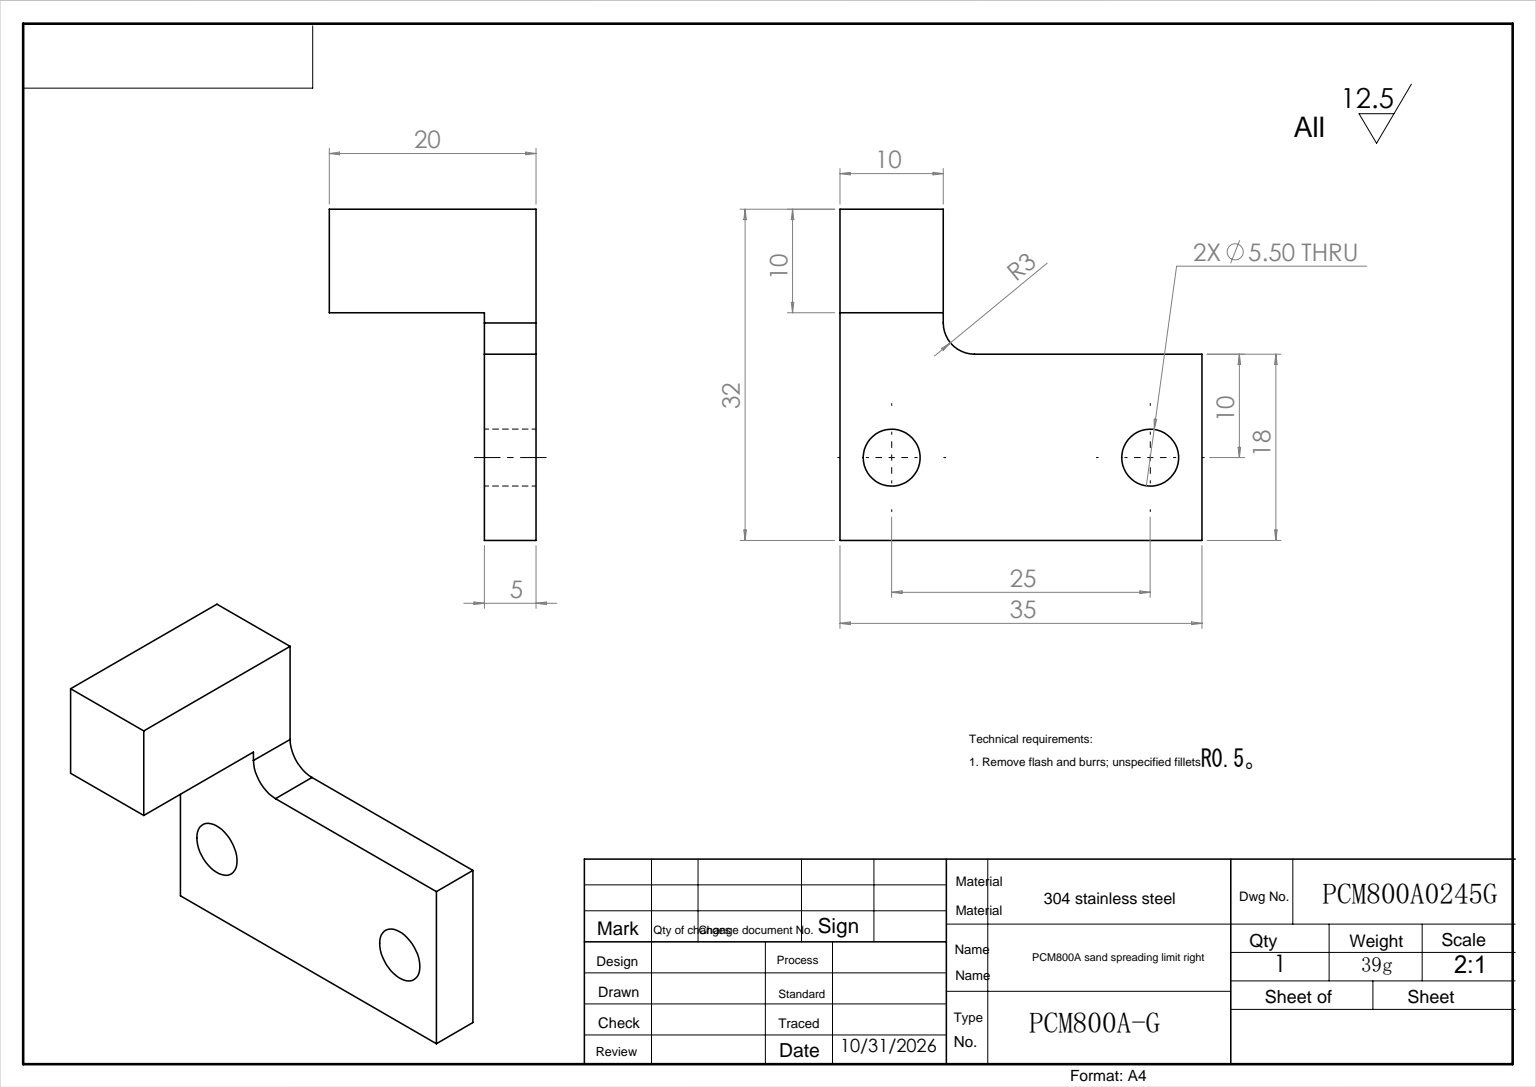
SolidWorks part; units mm, degrees
ref_plane "前视基准面" through (0, 0, 0) normal (0, 0, 1) x (1, 0, 0)
ref_plane "上视基准面" through (0, 0, 0) normal (0, 1, 0) x (1, 0, 0)
ref_plane "右视基准面" through (0, 0, 0) normal (1, 0, 0) x (0, 0, -1)
sketch "草图1" plane through (0, 0, 0) normal (0, 0, 1) x (1, 0, 0)
  line L1 (0, 0) -> (35, 0)
  line L2 (0, 0) -> (0, 22)
  line L3 (13, 18) -> (35, 18)
  line L4 (35, 0) -> (35, 18)
  line L7 (0, 22) -> (10, 22)
  line L8 (10, 21) -> (10, 22)
  arc A0 (13, 18) -> (10, 21) centre (13, 21) cw
  dimension "D4" = 3
  dimension "D1" = 18
  dimension "D2" = 35
  dimension "D3" = 22
  dimension "D5" = 10
  dimension "D6" = 1
extrude "凸台-拉伸1" add sketch "草图1" along normal blind 5
sketch "草图5" plane through (0, 0, 0) normal (0, 0, -1) x (-1, 0, 0)
  line L1 (0, 22) -> (-10, 22)
  line L2 (0, 22) -> (0, 32)
  line L3 (0, 32) -> (-10, 32)
  line L4 (-10, 22) -> (-10, 32)
  dimension "D1" = 10
  dimension "D2" = 10
extrude "凸台-拉伸3" add sketch "草图5" against normal blind 20
sketch "草图4" plane through (0, 0, 0) normal (0, 0, -1) x (-1, 0, 0)
  line L1 (-17.5, 0) -> (-17.5, 27.8202) construction
  line L2 (0, 0) -> (-35, 0) construction
  line L3 (0, 32) -> (-10, 32) construction
  circle A0 centre (-30, 8) radius 2.75
  circle A1 centre (-5, 8) radius 2.75
  dimension "D3" = 25
  dimension "D5" = 5.5
  dimension "D6" = 5.5
  dimension "D1" = 24
  dimension "D2" = 24
  dimension "D4" = 12.5
extrude "切除-拉伸1" cut sketch "草图4" against normal blind 20
